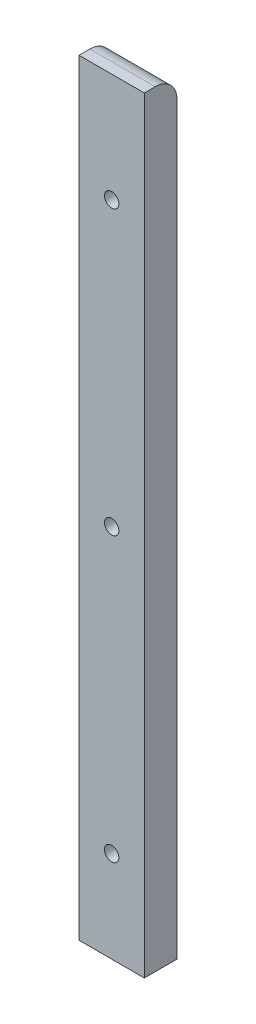
SolidWorks part; units mm, degrees
material "白色POM"
ref_plane "前基準面" through (0, 0, 0) normal (0, 0, 1) x (1, 0, 0)
ref_plane "上基準面" through (0, 0, 0) normal (0, 1, 0) x (1, 0, 0)
ref_plane "右基準面" through (0, 0, 0) normal (1, 0, 0) x (0, 0, -1)
sketch "草图1" plane through (0, 0, 0) normal (0, 0, 1) x (1, 0, 0)
  line L1 (-15, 176) -> (15, 176)
  line L2 (-15, 176) -> (-15, -176)
  line L3 (-15, -176) -> (15, -176)
  line L4 (15, 176) -> (15, -176)
  line L5 (-15, 176) -> (15, -176) construction
  line L6 (-15, -176) -> (15, 176) construction
  point P0 (0, 0)
  dimension "D1" = 30
  dimension "D2" = 352
extrude "凸台-拉伸1" add sketch "草图1" along normal blind 15
hole_wizard "打孔尺寸(%根据)内六角圆柱头螺钉的类型1" positions "草图3" profile "草图2" counterbore size "M6" standard "GB" end condition through all
sketch "草图3" plane through (0, 0, 0) normal (0, 0, -1) x (-1, 0, 0)
  line L0 (0, 176) -> (0, 126) construction
  line L1 (-15, 176) -> (15, 176) construction
  point P0 (0, 126)
  point P2 (0, -4)
  point P4 (0, -134)
  dimension "D1" = 50
  dimension "D2" = 130
  dimension "D3" = 130
sketch "草图2" plane through (0, 126, 0) normal (1, 0, 0) x (0, 1, 0)
  line L0 (0, 0) -> (0, 15)
  line L1 (0, 15) -> (3.3, 15)
  line L3 (3.3, 15) -> (3.3, 6.8)
  line L4 (3.3, 6.8) -> (5.5, 6.8)
  line L5 (5.5, 6.8) -> (5.5, 0)
  line L7 (5.5, 0) -> (0, 0)
  line L11 (0, -6.35) -> (0, 107.95) construction
  dimension "通孔孔直径" = 6.6
  dimension "通孔孔深度" = 15
  dimension "柱形沉头孔直径" = 11
  dimension "柱形沉头孔深度" = 6.8
fillet "圆角1" radius 10 1 edges at (0, 176, 0)
